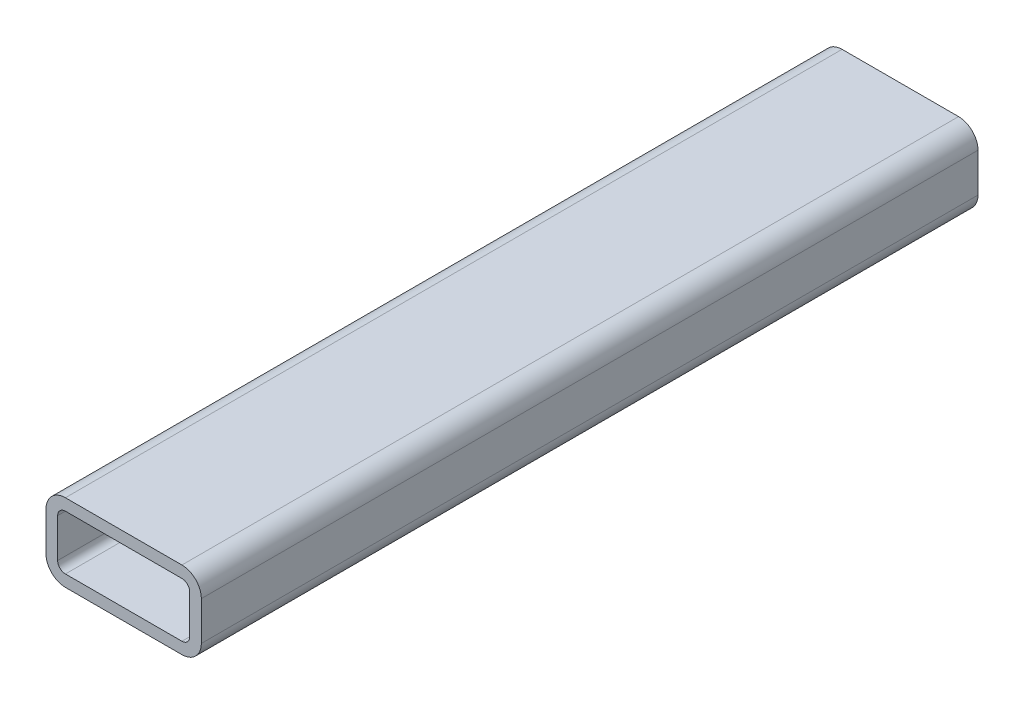
from build123d import *

# Parameters (mm, degrees)
BOSS_EXTRUDE1_DEPTH = 200


with BuildPart() as part:
    # Sketch1 → Boss-Extrude1 (new body)
    with BuildSketch(Plane.XY):
        with BuildLine():
            Line((5, 0), (35, 0))
            ThreePointArc((35, 0), (38.535533906, 1.464466094), (40, 5))
            Line((40, 5), (40, 15))
            ThreePointArc((40, 15), (38.535533906, 18.535533906), (35, 20))
            Line((35, 20), (5, 20))
            ThreePointArc((5, 20), (1.464466094, 18.535533906), (0, 15))
            Line((0, 15), (0, 5))
            ThreePointArc((0, 5), (1.464466094, 1.464466094), (5, 0))
        make_face()
        with BuildLine():
            Line((5, 17), (35, 17))
            ThreePointArc((35, 17), (36.414213562, 16.414213562), (37, 15))
            Line((37, 15), (37, 5))
            ThreePointArc((37, 5), (36.414213562, 3.585786438), (35, 3))
            Line((35, 3), (5, 3))
            ThreePointArc((5, 3), (3.585786438, 3.585786438), (3, 5))
            Line((3, 5), (3, 15))
            ThreePointArc((3, 15), (3.585786438, 16.414213562), (5, 17))
        make_face(mode=Mode.SUBTRACT)
    extrude(amount=BOSS_EXTRUDE1_DEPTH)


solid = part.part
